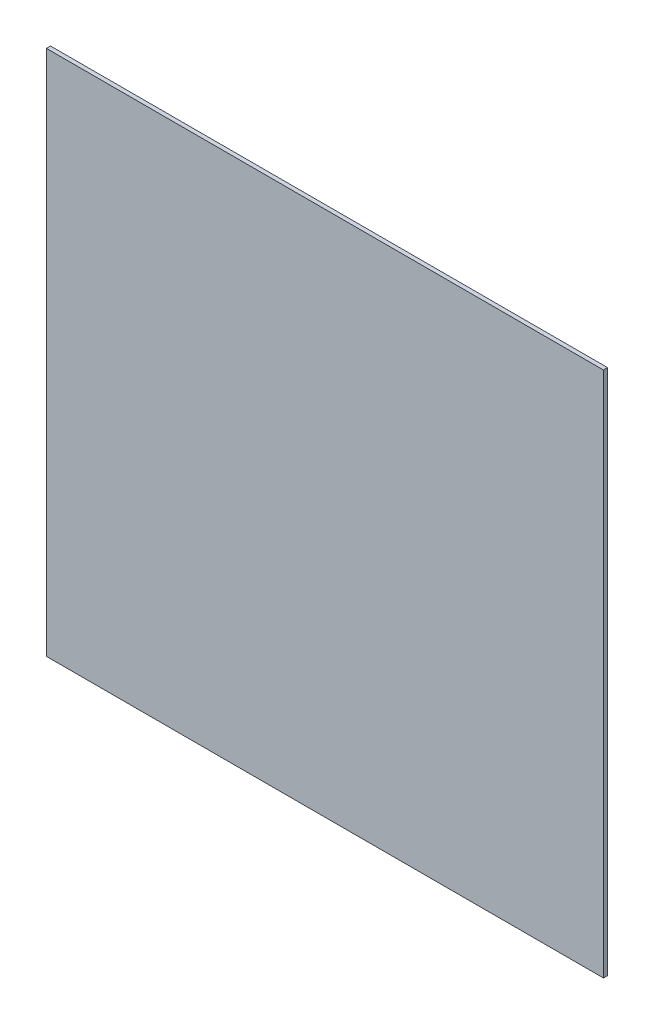
SolidWorks part; units mm, degrees
material "PMMA(有机玻璃)"
ref_plane "前视" through (0, 0, 0) normal (0, 0, 1) x (1, 0, 0)
ref_plane "上视" through (0, 0, 0) normal (0, 1, 0) x (1, 0, 0)
ref_plane "右视" through (0, 0, 0) normal (1, 0, 0) x (0, 0, -1)
sketch "草图1" plane through (0, 0, 0) normal (0, 0, 1) x (1, 0, 0)
  line L1 (-338, 319.5) -> (338, 319.5)
  line L2 (-338, 319.5) -> (-338, -319.5)
  line L3 (-338, -319.5) -> (338, -319.5)
  line L4 (338, 319.5) -> (338, -319.5)
  line L5 (-338, 319.5) -> (338, -319.5) construction
  line L6 (-338, -319.5) -> (338, 319.5) construction
  point P0 (0, 0)
  dimension "D1" = 639
  dimension "D2" = 676
extrude "凸台-拉伸1" add sketch "草图1" along normal blind 5
